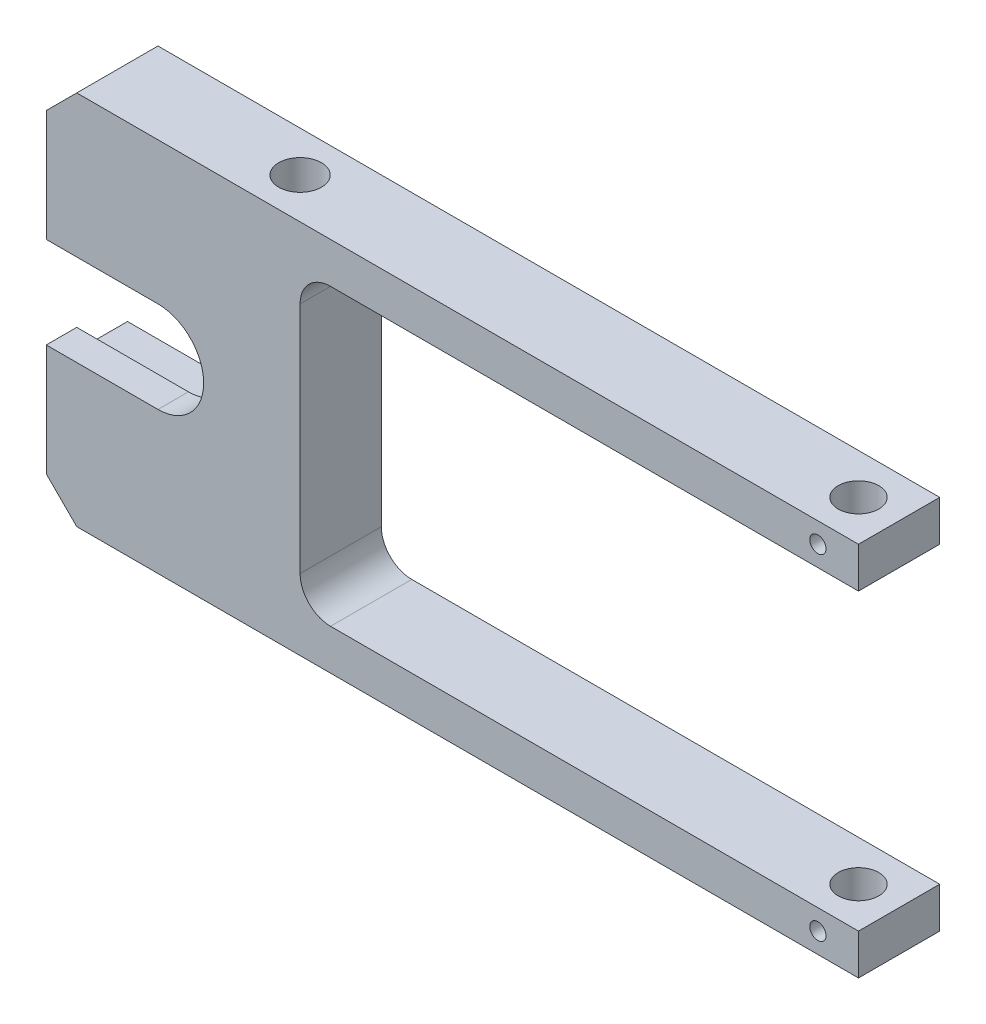
from build123d import *

# Parameters (mm, degrees)
EXTRUDE_1_DEPTH         = 4
CUT_EXTRUDE_1_REACH     = 68.408
SKETCH_2_R              = 2
CUT_EXTRUDE_2_REACH     = 68.408
SKETCH_3_R              = 2.1
HOLE_WIZARD_M2_1_REACH  = 86.054
HOLE_WIZARD_M2_1_BORE_R = 0.8
CUT_EXTRUDE_3_REACH     = 60.577
CUT_EXTRUDE_4_DEPTH     = 5
FILLET_1_R              = 3
CHAMFER_1_SIZE          = 3


with BuildPart() as part:
    # 草图1 → 凸台-拉伸1 (new, symmetric)
    with BuildSketch(Plane.XY):
        Polygon((0, 0), (0, 14.5), (55, 14.5), (55, 18.5), (-25, 18.5), (-25, -18.5), (55, -18.5), (55, -14.5), (0, -14.5), align=None)
    extrude(amount=EXTRUDE_1_DEPTH, both=True)

    # 切除-拉伸1: up to this face of the body (flat: up to its plane)
    cut_extrude_1_end = Plane(part.part.faces().sort_by_distance((15, -18.5, 0))[0])
    # 草图2 → 切除-拉伸1 (cut, up to the picked face)
    with BuildSketch(Plane(origin=(0, 18.5, 0), x_dir=(1, 0, 0), z_dir=(0, 1, 0)), mode=Mode.PRIVATE) as cut_extrude_1_sk1:
        with Locations(Location((51, 0, 0), (0, 0, 180))):
            Circle(SKETCH_2_R)
    cut_extrude_1_tool1 = split(extrude(cut_extrude_1_sk1.sketch, amount=-CUT_EXTRUDE_1_REACH, mode=Mode.PRIVATE), bisect_by=cut_extrude_1_end, keep=Keep.BOTH, mode=Mode.PRIVATE)
    add(cut_extrude_1_tool1.solids().sort_by(Axis((51, 18.5, 0), (0, -1, 0)))[0], mode=Mode.SUBTRACT)

    # 草图3 → 切除-拉伸2 (cut, up to next)
    with BuildSketch(Plane.XZ.offset(18.5), mode=Mode.PRIVATE) as cut_extrude_2_sk1:
        with Locations(Location((-4, 0, 0), (0, 0, 270))):
            Circle(SKETCH_3_R)
    cut_extrude_2_tool1 = extrude(cut_extrude_2_sk1.sketch, amount=-CUT_EXTRUDE_2_REACH, mode=Mode.PRIVATE) & part.part
    add(cut_extrude_2_tool1.solids().sort_by_distance((-4, -18.5, 0))[0], mode=Mode.SUBTRACT)

    # M2 螺纹孔1 bore (on position points) → M2 螺纹孔1 (cut, up to next)
    with BuildSketch(Plane(origin=(51, -16.5, 4), x_dir=(1, 0, 0), z_dir=(0, 0, 1)), mode=Mode.PRIVATE) as hole_wizard_m2_1_sk1:
        Circle(HOLE_WIZARD_M2_1_BORE_R)
    hole_wizard_m2_1_tool1 = extrude(hole_wizard_m2_1_sk1.sketch, amount=-HOLE_WIZARD_M2_1_REACH, mode=Mode.PRIVATE) & part.part
    hole_wizard_m2_1 = hole_wizard_m2_1_tool1.solids().sort_by_distance((51, -16.5, 4))[0]
    add(hole_wizard_m2_1, mode=Mode.SUBTRACT)

    # 镜向1: M2 螺纹孔1 across plane
    add(hole_wizard_m2_1.mirror(Plane.ZX), mode=Mode.SUBTRACT)

    # 草图5 → 切除-拉伸3 (cut, up to next)
    with BuildSketch(Plane.XY.offset(4), mode=Mode.PRIVATE) as cut_extrude_3_sk1:
        with BuildLine():
            Line((-25, 4.5), (-14, 4.5))
            ThreePointArc((-14, 4.5), (-9.5, 0), (-14, -4.5))
            Line((-14, -4.5), (-25, -4.5))
            Line((-25, -4.5), (-25, 4.5))
        make_face()
    cut_extrude_3_tool1 = extrude(cut_extrude_3_sk1.sketch, amount=-CUT_EXTRUDE_3_REACH, mode=Mode.PRIVATE) & part.part
    add(cut_extrude_3_tool1.solids().sort_by_distance((-17.698151, 0, 4))[0], mode=Mode.SUBTRACT)

    # 草图6 → 切除-拉伸4 (cut)
    with BuildSketch(Plane(origin=(0, 0, -4), x_dir=(-1, 0, 0), z_dir=(0, 0, -1))):
        with BuildLine():
            Line((25, -6.5), (25, 6.5))
            Line((25, 6.5), (14, 6.5))
            ThreePointArc((14, 6.5), (7.5, 0), (14, -6.5))
            Line((14, -6.5), (25, -6.5))
        make_face()
    extrude(amount=-CUT_EXTRUDE_4_DEPTH, mode=Mode.SUBTRACT)

    # 圆角1
    fillet_1_edges = [part.edges().sort_by_distance(p)[0] for p in [
        (0, -14.5, 0),
        (0, 14.5, 0),
    ]]
    fillet(fillet_1_edges, radius=FILLET_1_R)

    # 倒角1
    chamfer_1_edges = [part.edges().sort_by_distance(p)[0] for p in [
        (-25, -18.5, 0),
        (-25, 18.5, 0),
    ]]
    chamfer(chamfer_1_edges, length=CHAMFER_1_SIZE)


solid = part.part
